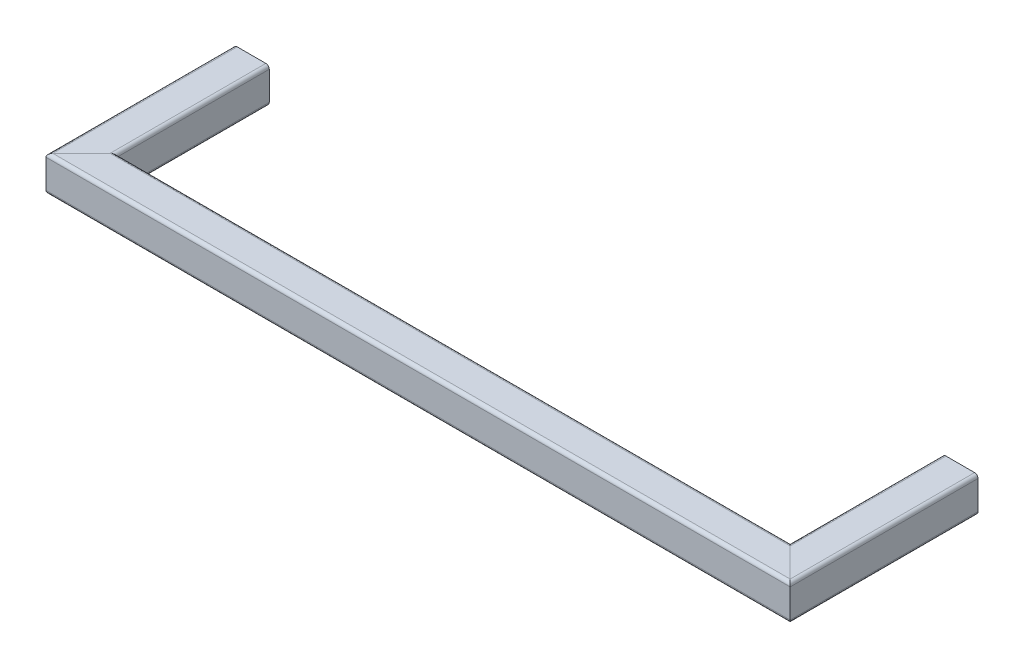
from build123d import *

# Parameters (mm, degrees)
GB_6728_1986_SQUARE_HOLLOW_SECTION_025_X_DEPTH    = 138.67766953
GB_6728_1986_SQUARE_HOLLOW_SECTION_0_3_DEPTH      = 537.355339059
GB_6728_1986_SQUARE_HOLLOW_SECTION_0_5_DEPTH      = 120
GB_6728_1986_SQUARE_HOLLOW_SECTION_0_5_DEPTH_BACK = 18.67766953
BOSS_EXTRUDE1_DEPTH                               = 3
SKETCH3_R                                         = 5
CUT_EXTRUDE1_DEPTH                                = 2


with BuildPart() as part:
    # Sketch11 on segment 1 (carried to segment 1) → Gb／6728-1986 square hollow section 025 X 25 X 1.2(1) (new body)
    with BuildSketch(Plane(origin=(250, 0, -120), x_dir=(1, 0, 0), z_dir=(0, 0, 1))):
        with BuildLine():
            Line((-10.1, -12.5), (10.1, -12.5))
            ThreePointArc((10.1, -12.5), (11.797056275, -11.797056275), (12.5, -10.1))
            Line((12.5, -10.1), (12.5, 10.1))
            ThreePointArc((12.5, 10.1), (11.797056275, 11.797056275), (10.1, 12.5))
            Line((10.1, 12.5), (-10.1, 12.5))
            ThreePointArc((-10.1, 12.5), (-11.797056275, 11.797056275), (-12.5, 10.1))
            Line((-12.5, 10.1), (-12.5, -10.1))
            ThreePointArc((-12.5, -10.1), (-11.797056275, -11.797056275), (-10.1, -12.5))
        make_face()
        with BuildLine():
            Line((-10.1, -11.3), (10.1, -11.3))
            ThreePointArc((10.1, -11.3), (10.948528137, -10.948528137), (11.3, -10.1))
            Line((11.3, -10.1), (11.3, 10.1))
            ThreePointArc((11.3, 10.1), (10.948528137, 10.948528137), (10.1, 11.3))
            Line((10.1, 11.3), (-10.1, 11.3))
            ThreePointArc((-10.1, 11.3), (-10.948528137, 10.948528137), (-11.3, 10.1))
            Line((-11.3, 10.1), (-11.3, -10.1))
            ThreePointArc((-11.3, -10.1), (-10.948528137, -10.948528137), (-10.1, -11.3))
        make_face(mode=Mode.SUBTRACT)
    extrude(amount=GB_6728_1986_SQUARE_HOLLOW_SECTION_025_X_DEPTH)

    # Gb_6728-1986 square hollow section 0 2
    split(bisect_by=Plane(origin=(250, 0, 0), x_dir=(0, 1, 0), z_dir=(0.707106781, 0, -0.707106781)), keep=Keep.TOP)



with BuildPart() as body_2:
    # Sketch11 on segment 2 (carried to segment 2) → Gb_6728-1986 square hollow section 0 3 (new body)
    with BuildSketch(Plane.ZY.offset(-268.67766953)):
        with BuildLine():
            Line((-10.1, -12.5), (10.1, -12.5))
            ThreePointArc((10.1, -12.5), (11.797056275, -11.797056275), (12.5, -10.1))
            Line((12.5, -10.1), (12.5, 10.1))
            ThreePointArc((12.5, 10.1), (11.797056275, 11.797056275), (10.1, 12.5))
            Line((10.1, 12.5), (-10.1, 12.5))
            ThreePointArc((-10.1, 12.5), (-11.797056275, 11.797056275), (-12.5, 10.1))
            Line((-12.5, 10.1), (-12.5, -10.1))
            ThreePointArc((-12.5, -10.1), (-11.797056275, -11.797056275), (-10.1, -12.5))
        make_face()
        with BuildLine():
            Line((-10.1, -11.3), (10.1, -11.3))
            ThreePointArc((10.1, -11.3), (10.948528137, -10.948528137), (11.3, -10.1))
            Line((11.3, -10.1), (11.3, 10.1))
            ThreePointArc((11.3, 10.1), (10.948528137, 10.948528137), (10.1, 11.3))
            Line((10.1, 11.3), (-10.1, 11.3))
            ThreePointArc((-10.1, 11.3), (-10.948528137, 10.948528137), (-11.3, 10.1))
            Line((-11.3, 10.1), (-11.3, -10.1))
            ThreePointArc((-11.3, -10.1), (-10.948528137, -10.948528137), (-10.1, -11.3))
        make_face(mode=Mode.SUBTRACT)
    extrude(amount=GB_6728_1986_SQUARE_HOLLOW_SECTION_0_3_DEPTH)

    # Gb_6728-1986 square hollow section 0 3 m
    split(bisect_by=Plane(origin=(-250, 0, 0), x_dir=(0, 1, 0), z_dir=(0.707106781, 0, 0.707106781)), keep=Keep.TOP)

    # Gb_6728-1986 square hollow section 0 4
    split(bisect_by=Plane(origin=(250, 0, 0), x_dir=(0, -1, 0), z_dir=(-0.707106781, 0, 0.707106781)), keep=Keep.TOP)


with BuildPart() as body_3:
    # Sketch11 → Gb_6728-1986 square hollow section 0 5 (new, two sides: drawn at the far end of the back side and taken through both)
    with BuildSketch(Plane(origin=(-250, 0, 0), x_dir=(-1, 0, 0), z_dir=(0, 0, -1)).offset(-GB_6728_1986_SQUARE_HOLLOW_SECTION_0_5_DEPTH_BACK)):
        with BuildLine():
            Line((-10.1, -12.5), (10.1, -12.5))
            ThreePointArc((10.1, -12.5), (11.797056275, -11.797056275), (12.5, -10.1))
            Line((12.5, -10.1), (12.5, 10.1))
            ThreePointArc((12.5, 10.1), (11.797056275, 11.797056275), (10.1, 12.5))
            Line((10.1, 12.5), (-10.1, 12.5))
            ThreePointArc((-10.1, 12.5), (-11.797056275, 11.797056275), (-12.5, 10.1))
            Line((-12.5, 10.1), (-12.5, -10.1))
            ThreePointArc((-12.5, -10.1), (-11.797056275, -11.797056275), (-10.1, -12.5))
        make_face()
        with BuildLine():
            Line((-10.1, -11.3), (10.1, -11.3))
            ThreePointArc((10.1, -11.3), (10.948528137, -10.948528137), (11.3, -10.1))
            Line((11.3, -10.1), (11.3, 10.1))
            ThreePointArc((11.3, 10.1), (10.948528137, 10.948528137), (10.1, 11.3))
            Line((10.1, 11.3), (-10.1, 11.3))
            ThreePointArc((-10.1, 11.3), (-10.948528137, 10.948528137), (-11.3, 10.1))
            Line((-11.3, 10.1), (-11.3, -10.1))
            ThreePointArc((-11.3, -10.1), (-10.948528137, -10.948528137), (-10.1, -11.3))
        make_face(mode=Mode.SUBTRACT)
    extrude(amount=GB_6728_1986_SQUARE_HOLLOW_SECTION_0_5_DEPTH + GB_6728_1986_SQUARE_HOLLOW_SECTION_0_5_DEPTH_BACK)

    # Gb_6728-1986 square hollow section 0 5 m
    split(bisect_by=Plane(origin=(-250, 0, 0), x_dir=(0, -1, 0), z_dir=(-0.707106781, 0, -0.707106781)), keep=Keep.TOP)


with BuildPart() as part_1:
    add(part.part)

    add(body_3.part)  # Boss-Extrude1 merges body 3
    # Sketch2 → Boss-Extrude1 (add)
    with BuildSketch(Plane(origin=(0, 0, -120), x_dir=(-1, 0, 0), z_dir=(0, 0, -1))):
        with BuildLine():
            Line((-262.5, 10.1), (-262.5, -10.1))
            ThreePointArc((-262.5, -10.1), (-261.797056275, -11.797056275), (-260.1, -12.5))
            Line((-260.1, -12.5), (-239.9, -12.5))
            ThreePointArc((-239.9, -12.5), (-238.202943725, -11.797056275), (-237.5, -10.1))
            Line((-237.5, -10.1), (-237.5, 10.1))
            ThreePointArc((-237.5, 10.1), (-238.202943725, 11.797056275), (-239.9, 12.5))
            Line((-239.9, 12.5), (-260.1, 12.5))
            ThreePointArc((-260.1, 12.5), (-261.797056275, 11.797056275), (-262.5, 10.1))
        make_face()
        with BuildLine():
            Line((260.1, 12.5), (239.9, 12.5))
            ThreePointArc((239.9, 12.5), (238.202943725, 11.797056275), (237.5, 10.1))
            Line((237.5, 10.1), (237.5, -10.1))
            ThreePointArc((237.5, -10.1), (238.202943725, -11.797056275), (239.9, -12.5))
            Line((239.9, -12.5), (260.1, -12.5))
            ThreePointArc((260.1, -12.5), (261.797056275, -11.797056275), (262.5, -10.1))
            Line((262.5, -10.1), (262.5, 10.1))
            ThreePointArc((262.5, 10.1), (261.797056275, 11.797056275), (260.1, 12.5))
        make_face()
    extrude(amount=-BOSS_EXTRUDE1_DEPTH)

    # Sketch3 → Cut-Extrude1 (cut)
    with BuildSketch(Plane.XZ.offset(12.5)):
        with Locations(Location((250, -105, 0), (0, 0, 270))):
            Circle(SKETCH3_R)
        with Locations(Location((-250, -105, 0), (0, 0, 90))):
            Circle(SKETCH3_R)
    extrude(amount=-CUT_EXTRUDE1_DEPTH, mode=Mode.SUBTRACT)


solid = Compound([body_2.part, part_1.part])
